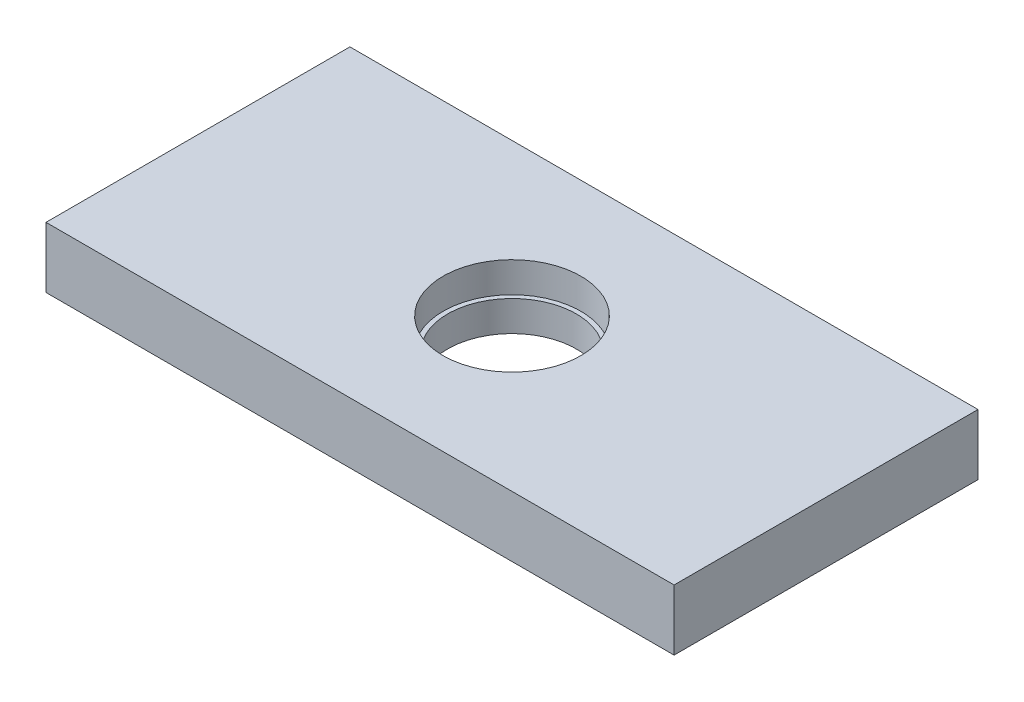
from build123d import *

# Parameters (mm, degrees)
SKETCH_1_W          = 310
SKETCH_1_H          = 150
EXTRUDE_1_DEPTH     = 30
SKETCH_2_R          = 31.75
CUT_EXTRUDE_1_DEPTH = 175.785582929
SKETCH_3_R          = 34
CUT_EXTRUDE_2_DEPTH = 15


with BuildPart() as part:
    # 草图1 → 凸台-拉伸1 (new body)
    with BuildSketch(Plane(origin=(0, 0, 0), x_dir=(1, 0, 0), z_dir=(0, 1, 0))):
        Rectangle(SKETCH_1_W, SKETCH_1_H)
    extrude(amount=EXTRUDE_1_DEPTH)

    # 草图2 → 切除-拉伸1 (cut, through all)
    with BuildSketch(Plane(origin=(0, 30, 0), x_dir=(1, 0, 0), z_dir=(0, 1, 0))):
        with Locations(Location((0, 0, 0), (0, 0, 270))):
            Circle(SKETCH_2_R)
    extrude(amount=-CUT_EXTRUDE_1_DEPTH, mode=Mode.SUBTRACT)

    # 草图3 → 切除-拉伸2 (cut)
    with BuildSketch(Plane(origin=(0, 30, 0), x_dir=(1, 0, 0), z_dir=(0, 1, 0))):
        with Locations(Location((0, 0, 0), (0, 0, 270))):
            Circle(SKETCH_3_R)
    extrude(amount=-CUT_EXTRUDE_2_DEPTH, mode=Mode.SUBTRACT)


solid = part.part
